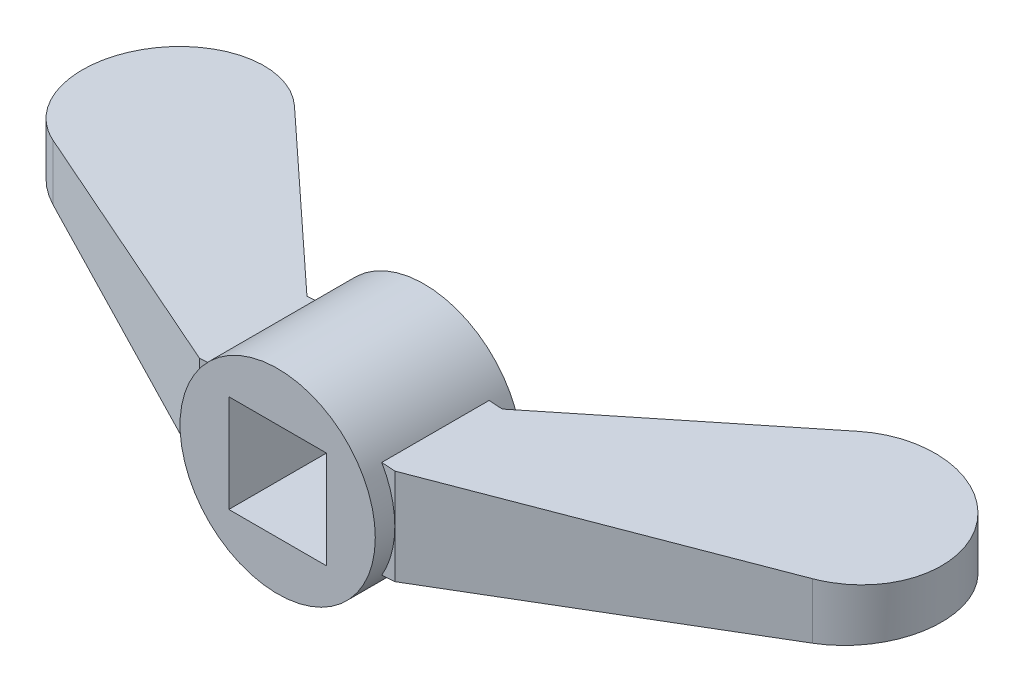
from build123d import *

# Parameters (mm, degrees)
SKETCH1_R           = 10
SKETCH1_W           = 10
SKETCH1_H           = 10
BOSS_EXTRUDE1_DEPTH = 7.5
SKETCH2_R           = 9
BOSS_EXTRUDE2_DEPTH = 5
CUT_EXTRUDE1_DEPTH  = 38


with BuildPart() as part:
    # Sketch1 → Boss-Extrude1 (new, symmetric)
    with BuildSketch(Plane.XY):
        Circle(SKETCH1_R)
        Rectangle(SKETCH1_W, SKETCH1_H, mode=Mode.SUBTRACT)
    extrude(amount=BOSS_EXTRUDE1_DEPTH, both=True)

    # Sketch2 → Boss-Extrude2 (add, symmetric)
    with BuildSketch(Plane(origin=(0, 0, 0), x_dir=(1, 0, 0), z_dir=(0, 1, 0))):
        with Locations((-35, 16.5)):
            Circle(SKETCH2_R)
        with BuildLine():
            Line((-10, 5.5), (-28.863308582, 23.083389586))
            ThreePointArc((-28.863308582, 23.083389586), (-26.746812047, 20.089552705), (-26, 16.5))
            ThreePointArc((-26, 16.5), (-30.208648574, 8.881407511), (-38.898433669, 8.388143558))
            Line((-38.898433669, 8.388143558), (-10, -5.5))
            Line((-10, -5.5), (-8, -5.5))
            Line((-8, -5.5), (-8, 5.5))
            Line((-8, 5.5), (-10, 5.5))
        make_face()
    boss_extrude2 = extrude(amount=BOSS_EXTRUDE2_DEPTH, both=True)

    # Sketch3 → Cut-Extrude1 (cut, symmetric)
    with BuildSketch(Plane.XY):
        Polygon((-51.292921798, 13.040521839), (-8.660254038, 5), (-44, 2.5), align=None)
        Polygon((-44, -2.5), (-51.292921798, -11.445050359), (-8.660254038, -5), align=None)
    cut_extrude1 = extrude(amount=CUT_EXTRUDE1_DEPTH, both=True, mode=Mode.SUBTRACT)

    # Mirror1: Boss-Extrude2, Cut-Extrude1 across plane
    add(boss_extrude2.mirror(Plane(origin=(0, 0, 0), x_dir=(0, 0, 1), z_dir=(1, 0, 0))))
    add(cut_extrude1.mirror(Plane(origin=(0, 0, 0), x_dir=(0, 0, 1), z_dir=(1, 0, 0))), mode=Mode.SUBTRACT)


solid = part.part
